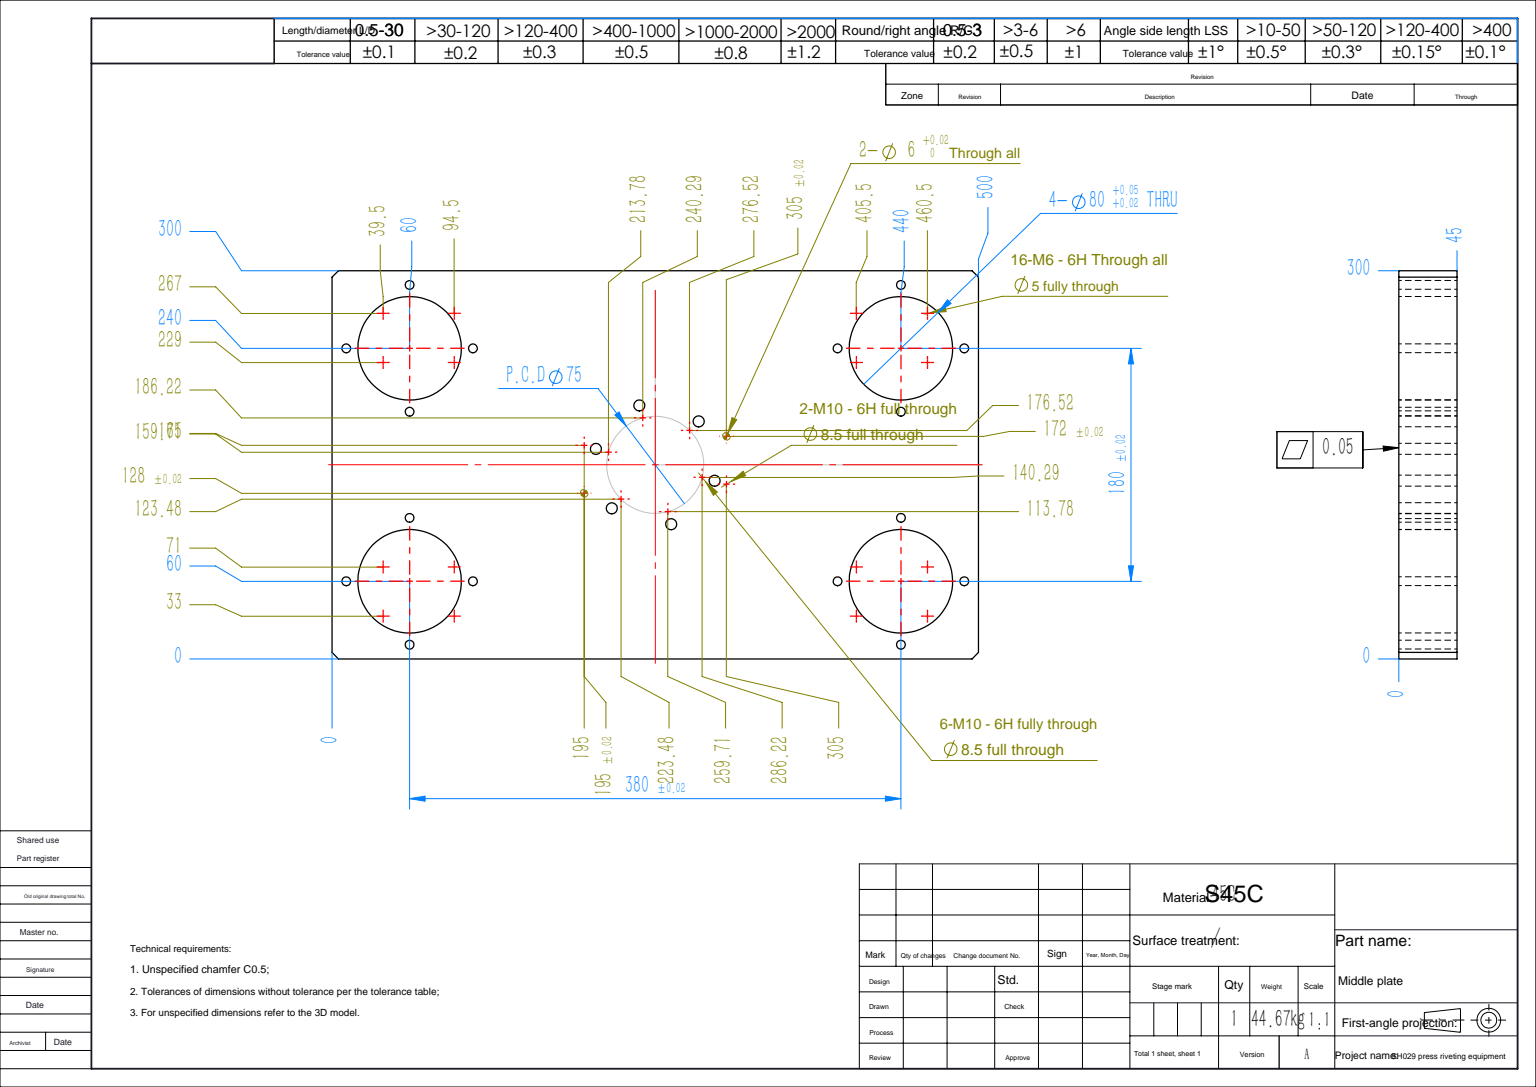
from build123d import *

# Parameters (mm, degrees)
SKETCH_1_W          = 500
SKETCH_1_H          = 300
EXTRUDE_1_DEPTH     = 45
CHAMFER_1_SIZE      = 5
SKETCH_6_R          = 40
CUT_EXTRUDE_1_DEPTH = 296
HOLE_WIZARD_M10_3_D = 8.5
HOLE_WIZARD_M8_1_D  = 6.8


with BuildPart() as part:
    # 草图1 → 凸台-拉伸1 (new body)
    with BuildSketch(Plane(origin=(0, 0, 0), x_dir=(1, 0, 0), z_dir=(0, 1, 0))):
        Rectangle(SKETCH_1_W, SKETCH_1_H)
    extrude(amount=EXTRUDE_1_DEPTH)

    # 倒角1
    chamfer_1_edges = [part.edges().sort_by_distance(p)[0] for p in [
        (250, 22.5, 150),
        (-250, 22.5, 150),
        (-250, 22.5, -150),
        (250, 22.5, -150),
    ]]
    chamfer(chamfer_1_edges, length=CHAMFER_1_SIZE)

    # 草图6 → 切除-拉伸1 (cut, through all)
    with BuildSketch(Plane(origin=(0, 45, 0), x_dir=(1, 0, 0), z_dir=(0, 1, 0))):
        with Locations(Location((190, -90, 0), (0, 0, 270))):
            Circle(SKETCH_6_R)
        with Locations(Location((190, 90, 0), (0, 0, 270))):
            Circle(SKETCH_6_R)
        with Locations(Location((-190, 90, 0), (0, 0, 270))):
            Circle(SKETCH_6_R)
        with Locations(Location((-190, -90, 0), (0, 0, 270))):
            Circle(SKETCH_6_R)
    extrude(amount=-CUT_EXTRUDE_1_DEPTH, mode=Mode.SUBTRACT)

    # M10 螺纹孔3 (through all)
    with Locations(Plane(origin=(0, 45, 0), x_dir=(1, 0, 0), z_dir=(0, 1, 0))):
        with Locations((-12.293904642, 45.881476749), (-45.881476749, 12.293904642), (-33.587572106, -33.587572106), (12.293904642, -45.881476749), (45.881476749, -12.293904642), (33.587572106, 33.587572106)):
            Hole(HOLE_WIZARD_M10_3_D / 2)

    # M8 螺纹孔1 (through all)
    with Locations(Plane(origin=(0, 45, 0), x_dir=(1, 0, 0), z_dir=(0, 1, 0))):
        with Locations((239, -90), (190, -139), (141, -90), (190, -41), (239, 90), (190, 41), (141, 90), (190, 139), (-141, -90), (-190, -139), (-239, -90), (-190, -41), (-141, 90), (-190, 41), (-239, 90), (-190, 139)):
            Hole(HOLE_WIZARD_M8_1_D / 2)


solid = part.part
